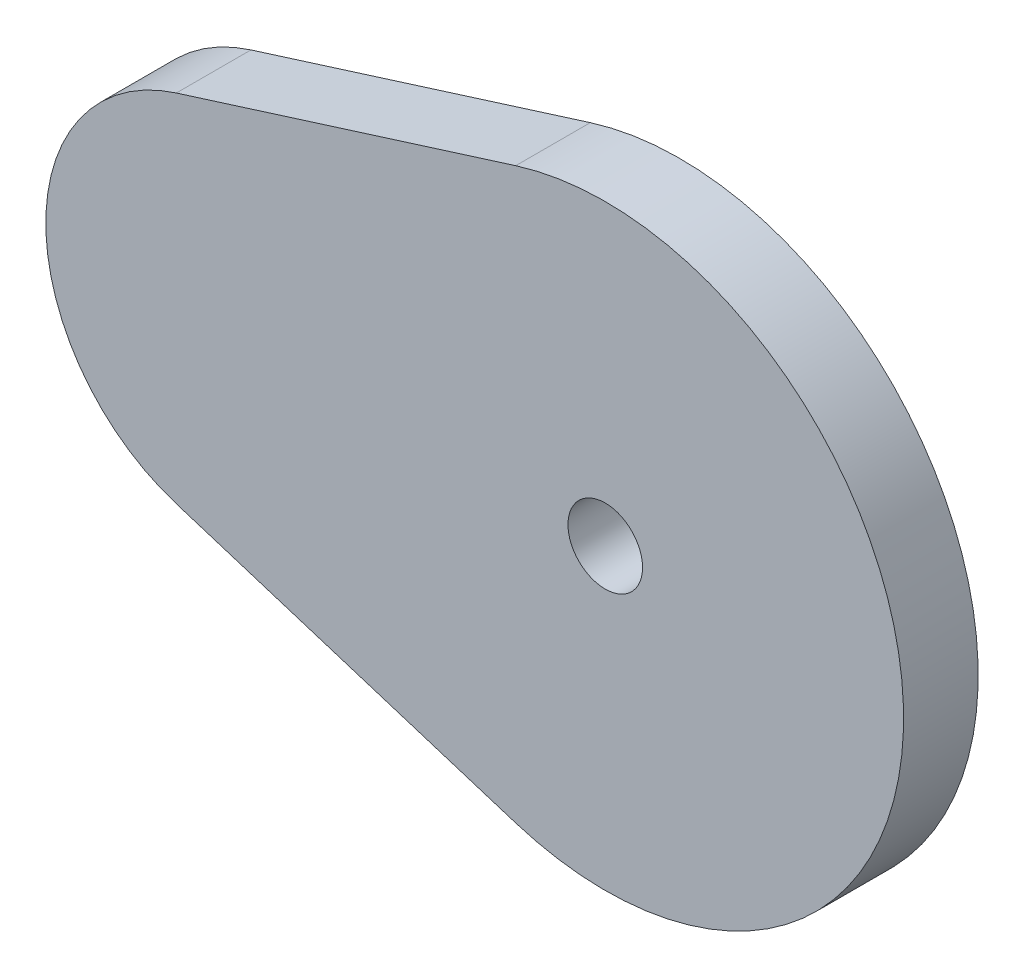
SolidWorks part; units mm, degrees
ref_plane "Front Plane" through (0, 0, 0) normal (0, 0, 1) x (1, 0, 0)
ref_plane "Top Plane" through (0, 0, 0) normal (0, 1, 0) x (1, 0, 0)
ref_plane "Right Plane" through (0, 0, 0) normal (1, 0, 0) x (0, 0, -1)
other "Configuration Table"
sketch "Sketch1" plane through (0, 0, 0) normal (0, 0, 1) x (1, 0, 0)
  line L0 (-57.5, 23.8485) -> (-12, 38.1576)
  line L1 (-57.5, -23.8485) -> (-12, -38.1576)
  arc A0 (-12, -38.1576) -> (-12, 38.1576) centre (0, 0) ccw
  arc A1 (-57.5, 23.8485) -> (-57.5, -23.8485) centre (-50, 0) ccw
  circle A3 centre (0, 0) radius 5
  dimension "D1" = 80
  dimension "D2" = 50
  dimension "D3" = 50
  dimension "D4" = 10
extrude "Boss-Extrude1" add sketch "Sketch1" along normal blind 10
